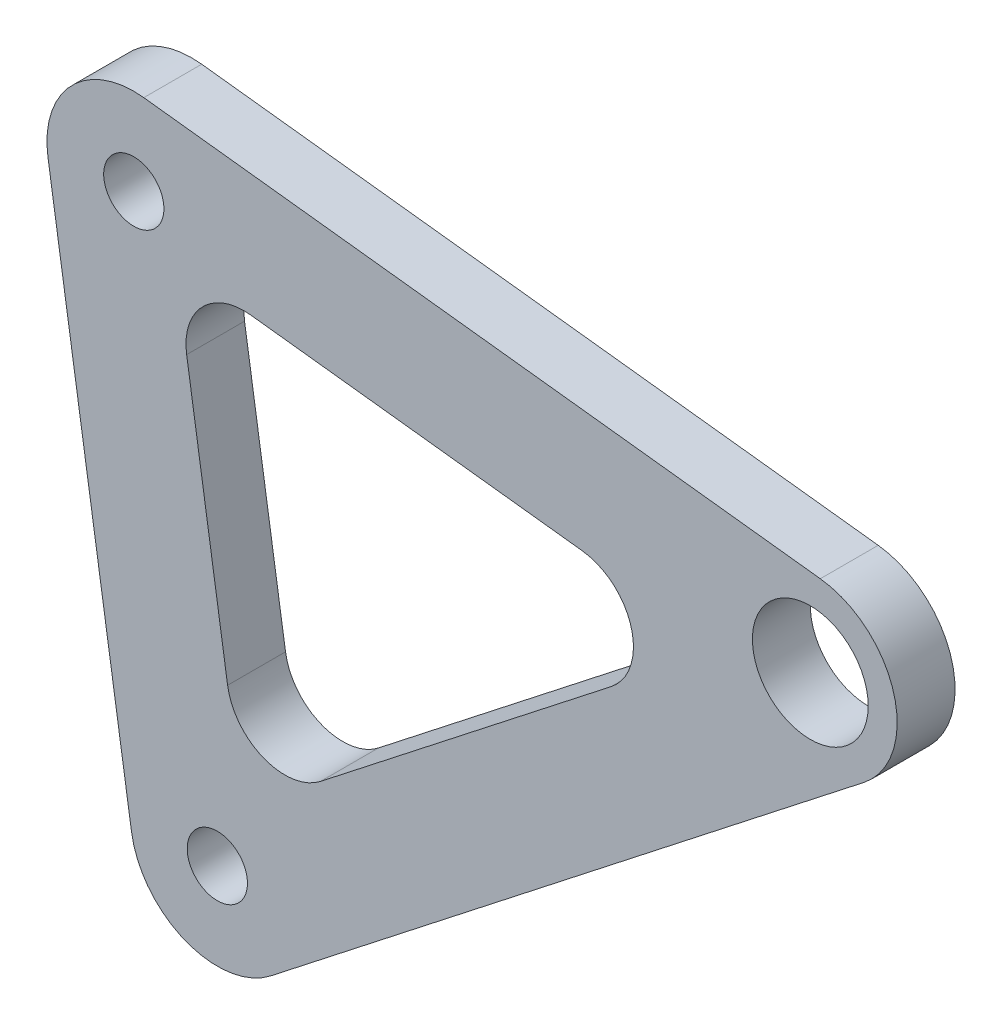
from build123d import *

# Parameters (mm, degrees)
SKETCH1_R           = 5
SKETCH1_R_2         = 2.6
BOSS_EXTRUDE1_DEPTH = 5


with BuildPart() as part:
    # Sketch1 → Boss-Extrude1 (new body)
    with BuildSketch(Plane.XY):
        with BuildLine():
            Line((-7.412562463, -1.141892169), (-0.198568318, -47.971342146))
            ThreePointArc((-0.198568318, -47.971342146), (4.453004984, -53.802751838), (11.835747448, -52.736174654))
            Line((11.835747448, -52.736174654), (63.035902792, -12.674296032))
            ThreePointArc((63.035902792, -12.674296032), (65.633751361, -4.735983598), (59.277288615, 0.682595814))
            Line((59.277288615, 0.682595814), (0.863139126, 7.450167169))
            ThreePointArc((0.863139126, 7.450167169), (-5.401815198, 5.202921542), (-7.412562463, -1.141892169))
        make_face()
        with Locations((58.414149489, -6.767571355)):
            Circle(SKETCH1_R, mode=Mode.SUBTRACT)
        with Locations((7.213994146, -46.829449977)):
            Circle(SKETCH1_R_2, mode=Mode.SUBTRACT)
        Circle(SKETCH1_R_2, mode=Mode.SUBTRACT)
        with BuildLine():
            Line((38.716618419, -7.505580332), (10.080053588, -4.187891081))
            ThreePointArc((10.080053588, -4.187891081), (5.903417372, -5.686054833), (4.562919195, -9.91593064))
            Line((4.562919195, -9.91593064), (8.099459791, -32.873289294))
            ThreePointArc((8.099459791, -32.873289294), (11.200508659, -36.760895756), (16.122336968, -36.049844299))
            Line((16.122336968, -36.049844299), (41.222361204, -16.410174896))
            ThreePointArc((41.222361204, -16.410174896), (42.95426025, -11.117966607), (38.716618419, -7.505580332))
        make_face(mode=Mode.SUBTRACT)
    extrude(amount=BOSS_EXTRUDE1_DEPTH)


solid = part.part
